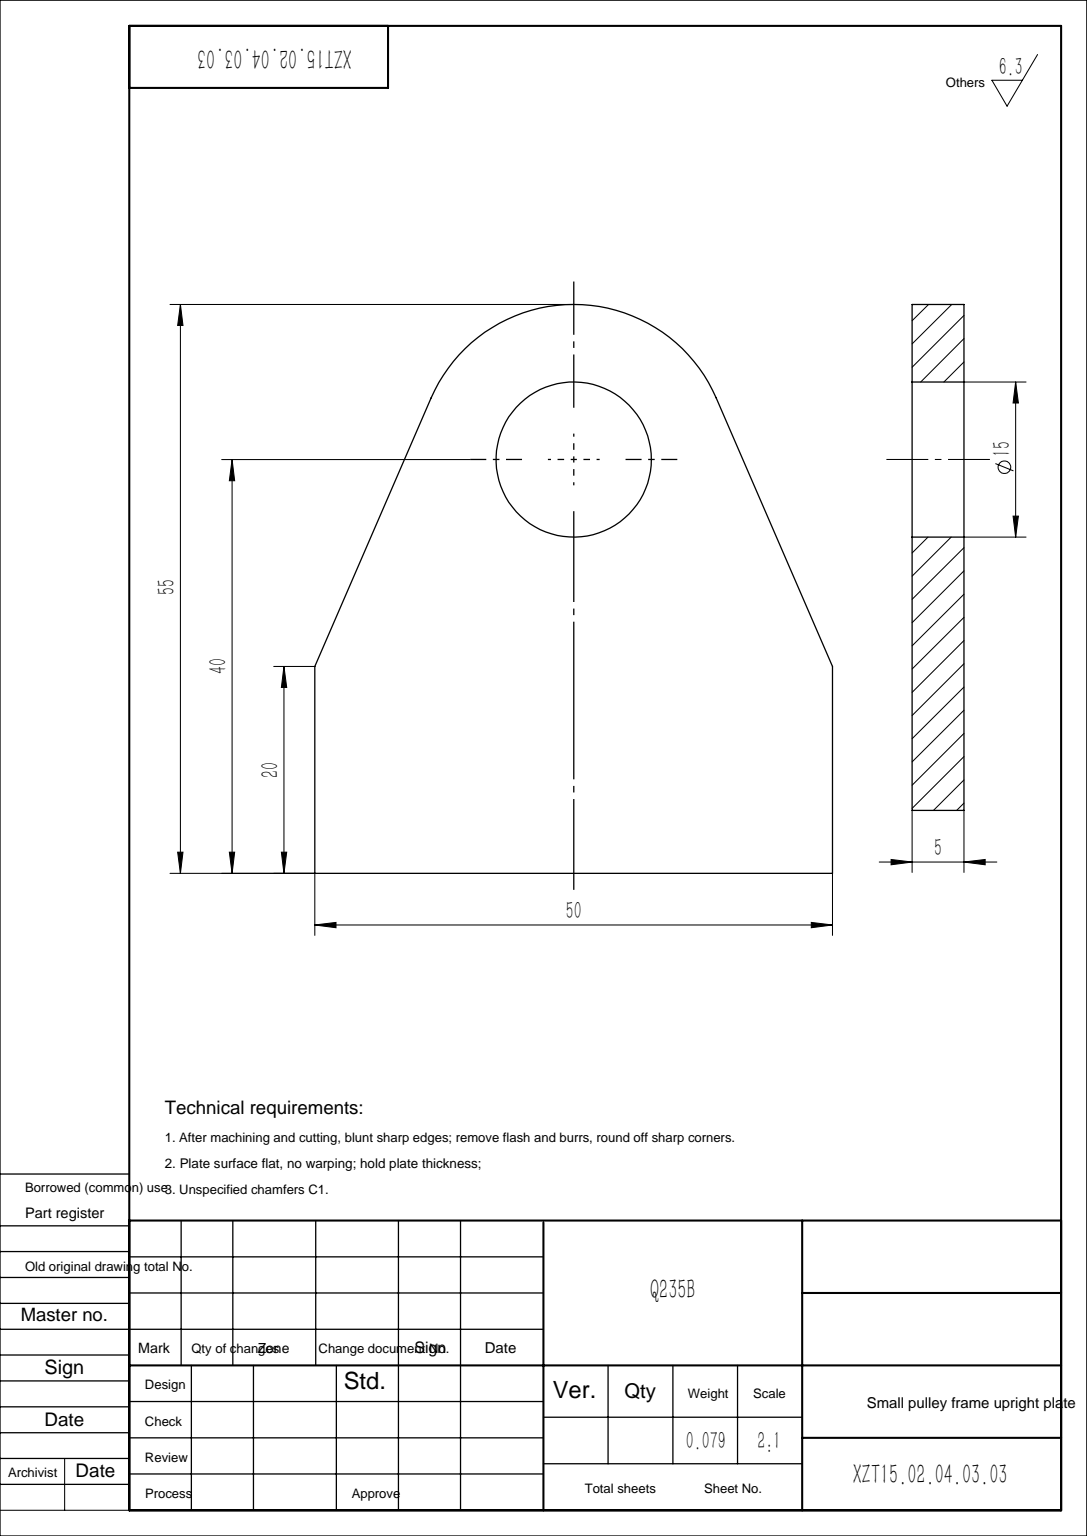
SolidWorks part; units mm, degrees
material "Q235B"
ref_plane "Front Plane" through (0, 0, 0) normal (0, 0, 1) x (1, 0, 0)
ref_plane "Top Plane" through (0, 0, 0) normal (0, 1, 0) x (1, 0, 0)
ref_plane "Right Plane" through (0, 0, 0) normal (1, 0, 0) x (0, 0, -1)
sketch "Sketch1" plane through (0, 0, 0) normal (0, 0, 1) x (1, 0, 0)
  line L0 (25, 0) -> (-25, 0)
  line L1 (-25, 0) -> (-13.7661, 25.9577)
  line L2 (0, 0) -> (0, 20) construction
  line L3 (25, 0) -> (13.7661, 25.9577)
  arc A0 (-13.7661, 25.9577) -> (13.7661, 25.9577) centre (0, 20) cw
  circle A1 centre (0, 20) radius 7.5
  dimension "D1" = 20
  dimension "D4" = 15
  dimension "D2" = 35
  dimension "D3" = 50
extrude "Boss-Extrude1" add sketch "Sketch1" along normal mid plane 5
sketch "Sketch2" plane through (0, 0, 2.5) normal (0, 0, 1) x (1, 0, 0)
  line L1 (-25, 0) -> (25, 0)
  line L2 (-25, 0) -> (-25, -20)
  line L3 (-25, -20) -> (25, -20)
  line L4 (25, 0) -> (25, -20)
  dimension "D1" = 20
extrude "Boss-Extrude2" add sketch "Sketch2" against normal blind 5
